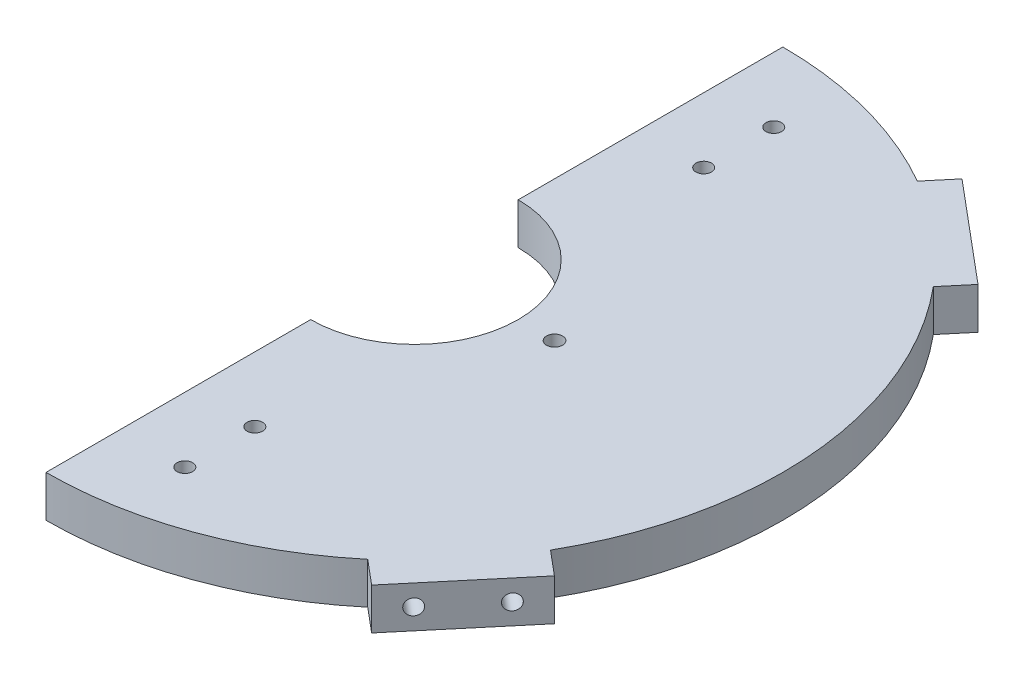
from build123d import *

# Parameters (mm, degrees)
BOSS_EXTRUDE1_DEPTH = 8
SKETCH2_R           = 1.5
CUT_EXTRUDE1_DEPTH  = 101.727354775
BOSS_EXTRUDE2_START = -71
SKETCH3_W           = 8
SKETCH3_H           = 25
BOSS_EXTRUDE2_DEPTH = 5
SKETCH4_R           = 1.5
CUT_EXTRUDE2_DEPTH  = 5
CIRPATTERN1_COUNT   = 2
CIRPATTERN1_ANGLE   = 90
SKETCH5_R           = 1.55
CUT_EXTRUDE3_DEPTH  = 101.727354775


with BuildPart() as part:
    # Sketch1 → Boss-Extrude1 (new body)
    with BuildSketch(Plane(origin=(0, 0, 0), x_dir=(1, 0, 0), z_dir=(0, 1, 0))):
        with BuildLine():
            Line((0, -71), (0, -20))
            ThreePointArc((0, -20), (20, 0), (0, 20))
            Line((0, 20), (0, 71))
            ThreePointArc((0, 71), (71, 0), (0, -71))
        make_face()
    extrude(amount=BOSS_EXTRUDE1_DEPTH)

    # Sketch2 → Cut-Extrude1 (cut, through all)
    with BuildSketch(Plane(origin=(0, 8, 0), x_dir=(1, 0, 0), z_dir=(0, 1, 0))):
        with Locations(Location((12.5, 43.25, 0), (0, 0, 270))):
            Circle(SKETCH2_R)
        with Locations(Location((12.5, 56.75, 0), (0, 0, 270))):
            Circle(SKETCH2_R)
        with Locations(Location((12.5, -43.25, 0), (0, 0, 90))):
            Circle(SKETCH2_R)
        with Locations(Location((12.5, -56.75, 0), (0, 0, 90))):
            Circle(SKETCH2_R)
    extrude(amount=-CUT_EXTRUDE1_DEPTH, mode=Mode.SUBTRACT)

    # Sketch3 → Boss-Extrude2 (add, symmetric)
    with BuildSketch(Plane(origin=(0, 0, 0), x_dir=(0, -1, 0), z_dir=(-0.6427876096865403, 0, 0.7660444431189772)).offset(BOSS_EXTRUDE2_START)):
        with Locations((-4, 0)):
            Rectangle(SKETCH3_W, SKETCH3_H)
    boss_extrude2 = extrude(amount=BOSS_EXTRUDE2_DEPTH, both=True)

    # Sketch4 → Cut-Extrude2 (cut)
    with BuildSketch(Plane(origin=(48.851858336, 0, -58.219377677), x_dir=(-0.7660444431189772, 0, -0.6427876096865404), z_dir=(0.6427876096865403, 0, -0.7660444431189771))):
        with Locations((-6.75, 4)):
            Circle(SKETCH4_R)
        with Locations((6.75, 4)):
            Circle(SKETCH4_R)
    cut_extrude2 = extrude(amount=-CUT_EXTRUDE2_DEPTH, mode=Mode.SUBTRACT)

    # CirPattern1: Boss-Extrude2, Cut-Extrude2 ×2 about axis
    cirpattern1_axis = Axis((0, 0, 0), (0, -1, 0))
    add([boss_extrude2.rotate(cirpattern1_axis, i * CIRPATTERN1_ANGLE / (CIRPATTERN1_COUNT - 1)) for i in range(1, CIRPATTERN1_COUNT)])
    add([cut_extrude2.rotate(cirpattern1_axis, i * CIRPATTERN1_ANGLE / (CIRPATTERN1_COUNT - 1)) for i in range(1, CIRPATTERN1_COUNT)], mode=Mode.SUBTRACT)

    # Sketch5 → Cut-Extrude3 (cut, through all)
    with BuildSketch(Plane(origin=(0, 8, 0), x_dir=(1, 0, 0), z_dir=(0, 1, 0))):
        with Locations(Location((27, 0, 0), (0, 0, 270))):
            Circle(SKETCH5_R)
    extrude(amount=-CUT_EXTRUDE3_DEPTH, mode=Mode.SUBTRACT)


solid = part.part
